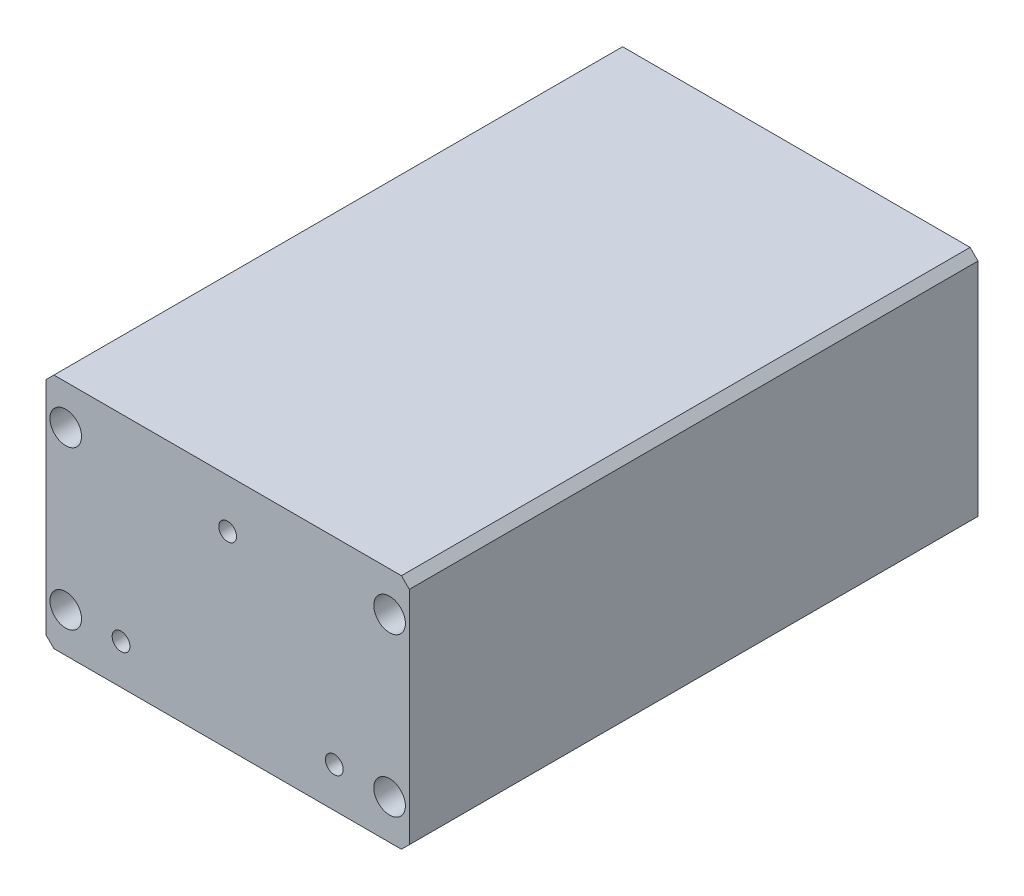
SolidWorks part; units mm, degrees
ref_plane "前视基准面" through (0, 0, 0) normal (0, 0, 1) x (1, 0, 0)
ref_plane "上视基准面" through (0, 0, 0) normal (0, 1, 0) x (1, 0, 0)
ref_plane "右视基准面" through (0, 0, 0) normal (1, 0, 0) x (0, 0, -1)
sketch "草图1" plane through (0, 0, 0) normal (0, 0, 1) x (1, 0, 0)
  line L1 (-46, 30) -> (46, 30)
  line L2 (-46, 30) -> (-46, -30)
  line L3 (-46, -30) -> (46, -30)
  line L4 (46, 30) -> (46, -30)
  line L5 (-46, 30) -> (46, -30) construction
  line L6 (-46, -30) -> (46, 30) construction
  point P0 (0, 0)
  dimension "D1" = 92
  dimension "D2" = 60
extrude "凸台-拉伸1" add sketch "草图1" along normal blind 144
hole_wizard "M4 六角凹头螺钉的柱形沉头孔1" positions "草图9" profile "草图10" counterbore size "M4" standard "ISO" end condition through all
sketch "草图9" plane through (0, 0, 144) normal (0, 0, 1) x (1, 0, 0)
  line L0 (-46, 0) -> (46, 0) construction
  line L1 (-46, 30) -> (-46, -30) construction
  line L2 (46, -30) -> (46, 30) construction
  line L4 (0, 30) -> (0, -30) construction
  line L5 (46, 30) -> (-46, 30) construction
  line L6 (-46, -30) -> (46, -30) construction
  point P0 (-41, 20)
  point P2 (-41, -20)
  point P4 (41, 20)
  point P6 (41, -20)
  dimension "D1" = 40
  dimension "D2" = 82
sketch "草图10" plane through (-41, 20, 144) normal (1, 0, 0) x (0, -1, 0)
  line L0 (0, 0) -> (0, 144)
  line L1 (0, 144) -> (2.25, 144)
  line L3 (2.25, 144) -> (2.25, 35)
  line L4 (2.25, 35) -> (4, 35)
  line L5 (4, 35) -> (4, 0)
  line L7 (4, 0) -> (0, 0)
  line L11 (0, -6.35) -> (0, 107.95) construction
  dimension "通孔孔直径" = 4.5
  dimension "通孔孔深度" = 144
  dimension "柱形沉头孔直径" = 8
  dimension "柱形沉头孔深度" = 35
chamfer "倒角1" distance 2 angle 45 4 edges at (46, -30, 72) (46, 30, 72) (-46, -30, 72) (-46, 30, 72)
hole_wizard "M4 六角凹头螺钉的柱形沉头孔2" positions "草图11" profile "草图13" counterbore size "M4" standard "ISO" end condition through all
sketch "草图11" plane through (0, 0, 0) normal (0, 0, -1) x (-1, 0, 0)
  circle A0 centre (0, 17.7) radius 1.65 construction
  circle A1 centre (27, -19.9) radius 1.65 construction
  circle A2 centre (-27, -19.9) radius 1.65 construction
  point P0 (0, 17.7)
  point P2 (-27, -19.9)
  point P4 (27, -19.9)
sketch "草图13" plane through (0, 17.7, 0) normal (1, 0, 0) x (0, 1, 0)
  line L0 (0, 0) -> (0, 144)
  line L1 (0, 144) -> (2.25, 144)
  line L3 (2.25, 144) -> (2.25, 37)
  line L4 (2.25, 37) -> (4, 37)
  line L5 (4, 37) -> (4, 0)
  line L7 (4, 0) -> (0, 0)
  line L11 (0, -6.35) -> (0, 107.95) construction
  dimension "通孔孔直径" = 4.5
  dimension "通孔孔深度" = 144
  dimension "柱形沉头孔直径" = 8
  dimension "柱形沉头孔深度" = 37
